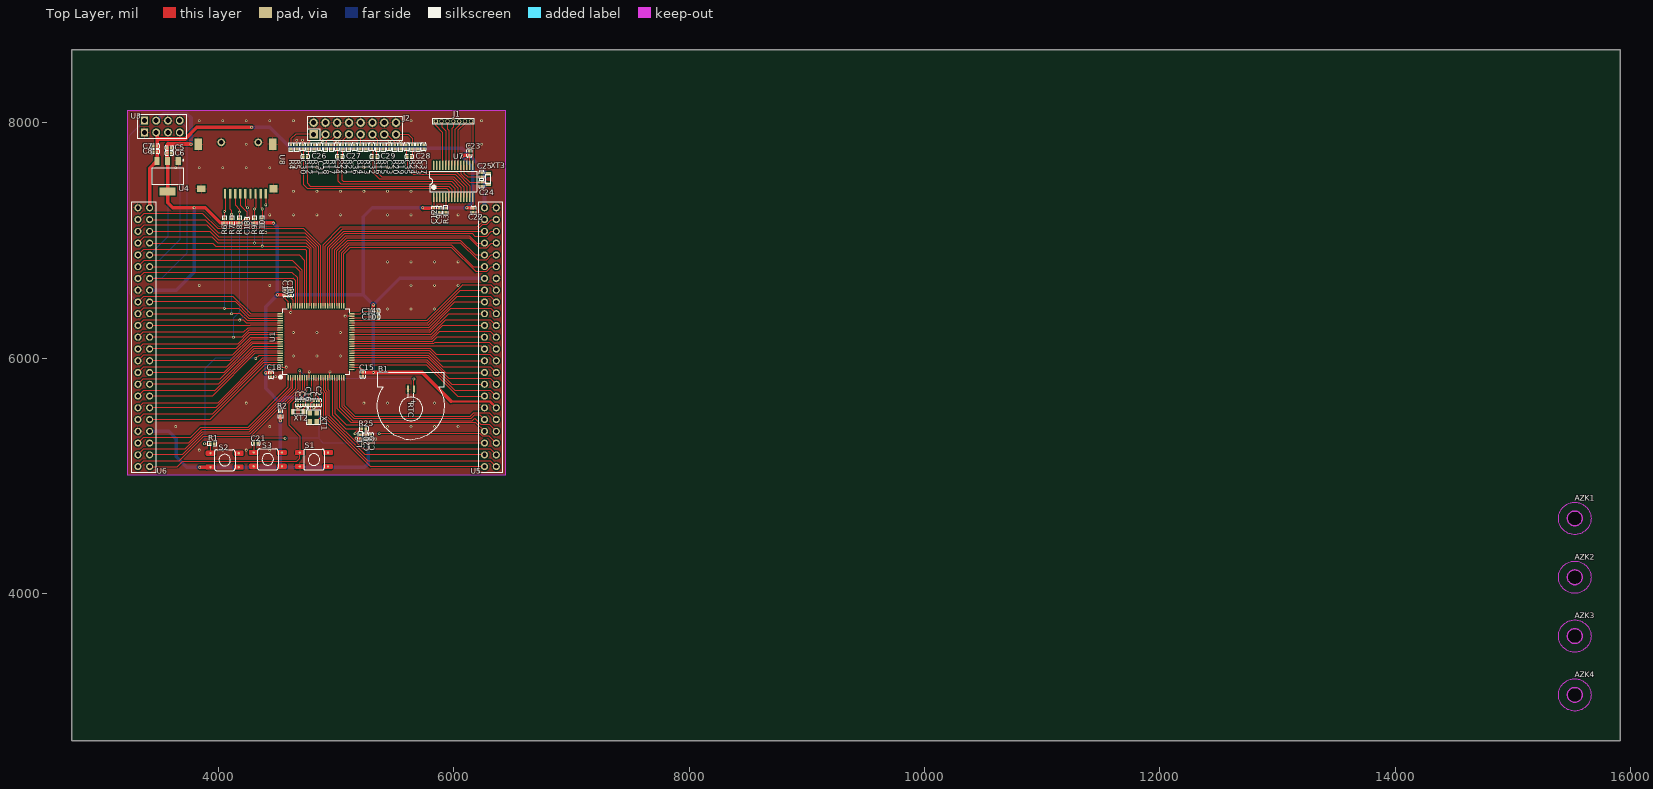
[diagram p0: Top Layer view]
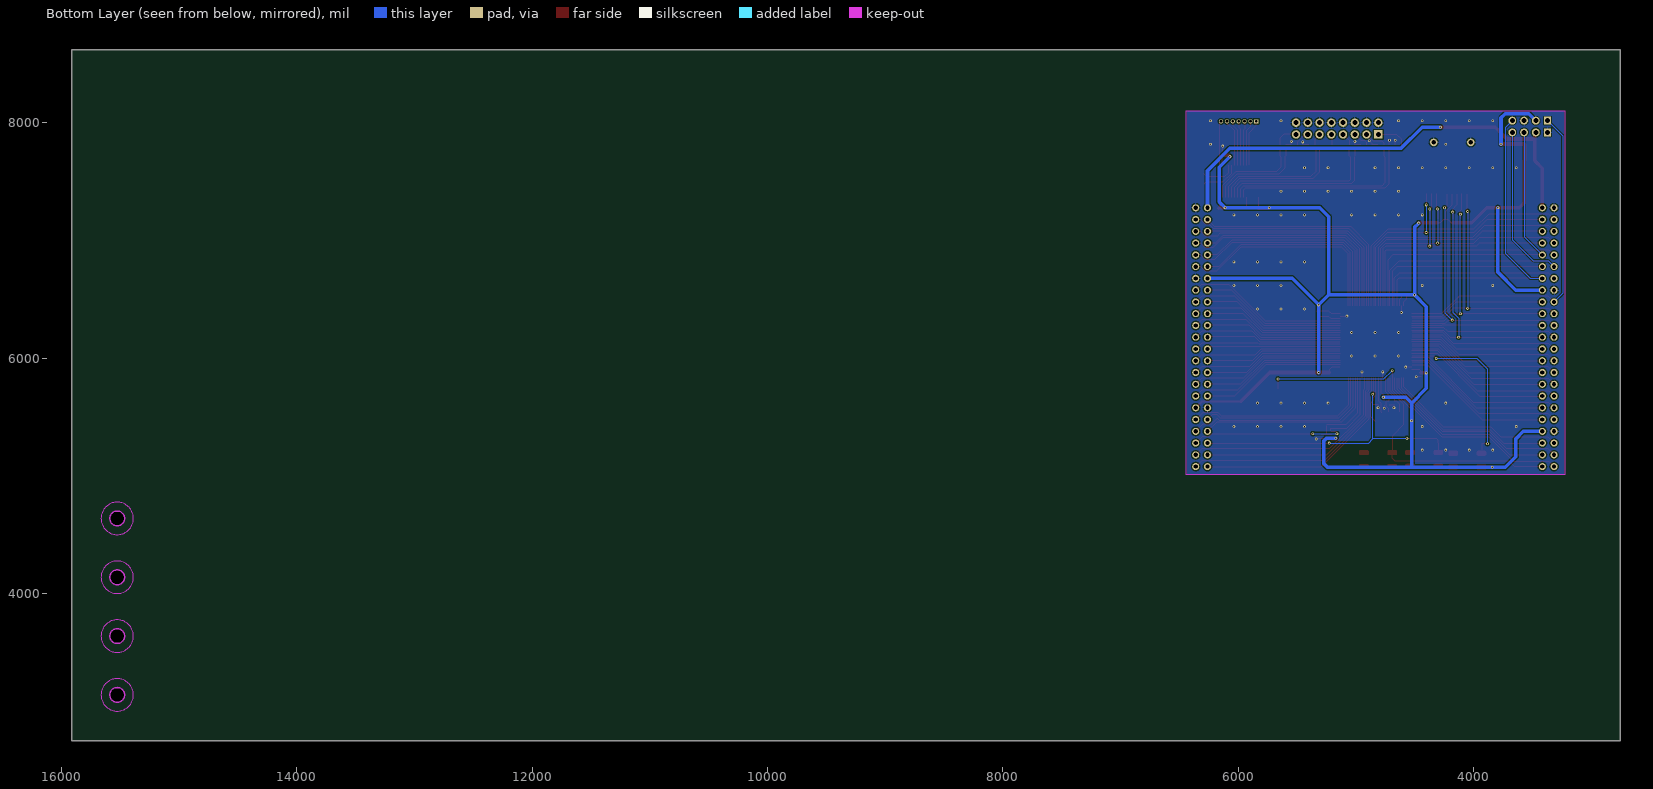
[diagram p1: Bottom Layer view, seen from below]
# Altium PCB MISC51975.pcbdoc
Units mil, origin at the board's own origin, x right, y up, seen from the top; angles counter-clockwise.
Board outline 13165.59 x 5873.19 mil, 2 copper layers (Top Layer, Bottom Layer), stack 2.757 mil thick; 83 components, 118 nets, 418 pads, 120 vias.

## Layer stack, top to bottom
Top Solder Mask Layer: solder mask 0.394, Dk 3.3
Top Layer: signal copper 1.379
Bottom Layer: signal copper 1.378
Bottom Solder Mask Layer: solder mask 0.394, Dk 3.3

## Board outline
15915.59,2750 2750,2750 2750,8623.19 15915.59,8623.19

## Design rules (kind name [scope] priority, off if disabled: settings)
BoardOutlineClearance Default_1 [All] p2: genericclearance=4 ignorepadtopadclearanceinfootprint=FALSE except(0: Arc-SplitContinuation Track-SplitContinuation SMDPad-SplitContinuation THPad-SplitContinuation Via-SplitContinuation Fill-SplitContinuation Region-SplitContinuation Poly-SplitContinuation Text-SplitContinuation Hole-SplitContinuation; 6: Arc-OutlineEdge Track-OutlineEdge SMDPad-OutlineEdge THPad-OutlineEdge Via-OutlineEdge Fill-OutlineEdge Region-OutlineEdge Poly-OutlineEdge Text-OutlineEdge Hole-OutlineEdge SMDPad-CutoutEdge THPad-CutoutEdge Via-CutoutEdge Fill-CutoutEdge Region-CutoutEdge Text-CutoutEdge; 6.9: Hole-CutoutEdge; 10: Poly-CutoutEdge; 11.8: Arc-CutoutEdge Track-CutoutEdge)
Clearance Default [All] p1: gap=4 ignorepadtopadclearanceinfootprint=FALSE except(6: SMDPad-Track SMDPad-SMDPad THPad-Track SMDPad-THPad THPad-THPad Track-Via SMDPad-Via THPad-Via Via-Via Fill-Track Region-Track Fill-SMDPad Region-SMDPad Fill-THPad Region-THPad Fill-Via Region-Via Fill-Fill Fill-Region Region-Region Arc-Track Arc-SMDPad Arc-THPad Arc-Via Fill-Arc Region-Arc Arc-Arc Text-Track SMDPad-Text Text-THPad Text-Via Fill-Text Region-Text Arc-Text Text-Text; 6.9: Hole-Track Hole-SMDPad Hole-THPad Hole-Via Fill-Hole Region-Hole Hole-Arc Hole-Text; 10: Poly-Track Poly-SMDPad Poly-THPad Poly-Via Poly-Fill Poly-Region Poly-Poly Poly-Arc Poly-Text Poly-Hole)
DiffPairsRouting differentialPair [All] p1: maxlimit=6 minlimit=5 mostfreqgap=6 toplayer_minwidth=5 toplayer_prefwidth=100 toplayer_maxwidth=100 toplayer_mingap=5 toplayer_prefgap=6 toplayer_maxgap=6 bottomlayer_minwidth=5 bottomlayer_prefwidth=100 bottomlayer_maxwidth=100 bottomlayer_mingap=5 bottomlayer_prefgap=6 bottomlayer_maxgap=6 maxuncoupledlength=10
HoleToHoleClearance otherClearance [All] p1: gap=11.8 allowstackedmicrovias=TRUE
Length netLength [All] p1: minlimit=0 maxlimit=0
MatchedLengths netLengthTolerance [All] p1: tolerance=1000
PasteMaskExpansion pasteMaskExpansion [All] p1: expansion=0
PlaneConnect innerPlane [All] p1: planeconnectstyle=Relief reliefexpansion=20 reliefentries=4 reliefconductorwidth=10 reliefairgap=10
PolygonConnect copperRegion [(InNet('GND'))] p1: connectstyle=Relief reliefconductorwidth=10 reliefentries=4 polygonreliefangle="90 Angle" airgapwidth=10 via.connectstyle=Relief via.reliefconductorwidth=10 via.reliefentries=4 via.polygonreliefangle="90 Angle" via.airgapwidth=10
RoutingVias Default_3 [All] p1: holewidth=12 width=24 viastyle="Through Hole" minholewidth=12 minwidth=24 maxholewidth=1181 maxwidth=1969
SolderMaskExpansion Common [IsVia] p1: expansion=-1000 istentingtop=TRUE
SolderMaskExpansion Common [All] p2: expansion=2 istentingtop=FALSE
Width Default_2 [All] p1: maxlimit=1000 minlimit=10 preferedwidth=10

## Components (designator, comment, footprint, x,y, rotation, side; value= is the part's Value field where it differs from the comment)
AZK1 "M3 mounting hole" M3安装孔(非金属化) 15527.8,4637.79 r0 top
AZK2 "M3 mounting hole" M3安装孔(非金属化) 15527.8,4137.79 r0 top
AZK3 "M3 mounting hole" M3安装孔(非金属化) 15527.8,3637.79 r0 top
AZK4 "M3 mounting hole" M3安装孔(非金属化) 15527.8,3137.79 r0 top
B1 "RTC" 焊盘引出RTC 5635.16,5567.96 r270 top
C1 "22pF" C0402 4808.14,5620.58 r90 top
C2 "22pF" C0402 4851.59,5621.23 r270 top
C3 "3pF" C0402 4673.14,5620.58 r270 top
C4 "3pF" C0402 4718.14,5620.58 r270 top
C5 "10uF" C0402 3580,7788.19 r180 top
C6 "10uF" C0402 3579.74,7741.59 r180 top
C7 "10uF" C0402 3459.74,7801.59 r180 top
C8 "100nF" C0402 3459.74,7756.59 r180 top
C9 "47uF" C0402 5875,7258.19 r90 top
C10 "100pF" C0402 5333.68,6351.39 r180 top
C11 "100pF" C0402 4613.68,6556.39 r270 top
C12 "100nF" C0402 5830,7258.19 r90 top
C13 "100pF" C0402 4240.52,7165.22 r90 top
C14 "100pF" C0402 5333.14,6400.58 r180 top
C15 "100pF" C0402 5225,5863.19 r90 top
C16 "100pF" C0402 4763.14,5620.58 r90 top
C17 "100pF" C0402 4568.14,6555.58 r270 top
C18 "100pF" C0402 4445,5858.19 r90 top
C19 "100pF" C0402 5293.66,5331.39 r90 top
C20 "10uF" C0402 5248.66,5330.88 r90 top
C21 "100nF" C0402 4316.73,5277.55 r180 top
C22 "47uF" C0402 6165,7258.19 r90 top
C23 "100nF" C0402 6130,7743.19 r270 top
C24 "47uF" C0402 6235,7478.19 r270 top
C25 "47uF" C0402 6235,7558.19 r90 top
C26 "10nF" C0402 4735,7713.19 r0 top
C27 "10nF" C0402 5030,7713.19 r0 top
C28 "10nF" C0402 5620,7713.19 r0 top
C29 "10nF" C0402 5325,7713.19 r0 top
C30 "1nF" C0402 4713.03,7795.67 r90 top
C31 "1nF" C0402 4860.1,7795.67 r90 top
C32 "1nF" C0402 5301.31,7795.67 r90 top
C33 "1nF" C0402 5448.38,7795.67 r90 top
C34 "1nF" C0402 5007.17,7795.67 r90 top
C35 "1nF" C0402 5595.45,7795.67 r90 top
C36 "1nF" C0402 5154.24,7795.67 r90 top
C37 "1nF" C0402 5742.52,7795.67 r90 top
J1 "1.27 pin header 7p" 1.27排针7P 6045,8013.19 r0 top
J2 "2.54 2*8P" HDR-TH_16P-P2.54-V-R2-C8-S2.54 5157.59,7952.11 r0 top
L1 "ferrite bead 600R" L0402 5203.14,5330.58 r90 top
R1 "10K" 贴片电阻0402封装 3945.92,5273.19 r0 top
R2 "200R" 贴片电阻0402封装 4525,5528.19 r90 top
R3 "0Ω" 贴片电阻0402封装 5930,7258.19 r90 top
R4 "100Ω" 贴片电阻0402封装 4615,7795.67 r270 top
R5 "10kΩ" 贴片电阻0402封装 4664,7795.67 r270 top
R6 "10K" 贴片电阻0402封装 4048.53,7167.99 r90 top
R7 "10K" 贴片电阻0402封装 4112.51,7167.99 r90 top
R8 "10K" 贴片电阻0402封装 4176.5,7167.99 r90 top
R9 "10K" 贴片电阻0402封装 4304.54,7167.99 r90 top
R10 "10K" 贴片电阻0402封装 4368.53,7167.99 r90 top
R11 "10kΩ" 贴片电阻0402封装 4811.07,7795.67 r270 top
R12 "100Ω" 贴片电阻0402封装 4762.07,7795.67 r270 top
R13 "10kΩ" 贴片电阻0402封装 5252.27,7795.67 r270 top
R14 "100Ω" 贴片电阻0402封装 5203.28,7795.67 r270 top
R15 "10kΩ" 贴片电阻0402封装 5399.34,7795.67 r270 top
R16 "100Ω" 贴片电阻0402封装 5350.35,7795.67 r270 top
R17 "10kΩ" 贴片电阻0402封装 4958.14,7795.67 r270 top
R18 "100Ω" 贴片电阻0402封装 4909.14,7795.67 r270 top
R19 "10kΩ" 贴片电阻0402封装 5546.41,7795.67 r270 top
R20 "100Ω" 贴片电阻0402封装 5497.42,7795.67 r270 top
R21 "10kΩ" 贴片电阻0402封装 5105.2,7795.67 r270 top
R22 "100Ω" 贴片电阻0402封装 5056.21,7795.67 r270 top
R23 "10kΩ" 贴片电阻0402封装 5693.48,7795.67 r270 top
R24 "100Ω" 贴片电阻0402封装 5644.49,7795.67 r270 top
R25 "0Ω" 贴片电阻0402封装 5233.14,5400.58 r180 top
S1 "K_USER" 按键开关4.5 4810,5138.19 r270 top
S2 "K_USER" 按键开关4.5 4051.41,5133.19 r270 top
S3 "K_USER" 按键开关4.5 4417.68,5139.98 r270 top
U1 "STM32H743VIT6" STM32H743VIT6 4828.14,6140.58 r90 top
U3 "HDR_2*4P" HDR_2*4P 3369.02,7919.17 r90 top
U4 "ASM1117" AMS1117-SOT-223 3566.29,7546.59 r180 top
U5 "STM32H7" 2*23 6310,6178.19 r180 top
U6 "STM32H7" 2*23 3363.54,6178.19 r180 top
U7 "ADS1256" SSOP-28_L10.2-W5.3-P0.65-LS7.8-BL 5994.95,7503.08 r0 top
U8 "MICRO SD TF card socket" "MICRO SD TF卡座" 4360.68,7507.71 r270 top
XT1 "XTAL3225" XTAL3225 4805,5498.19 r270 top
XT2 "32.768k" SMD-2012_2P 4675,5543.19 r0 top
XT3 "7.68MHz" SMD-2012_2P 6290,7523.19 r90 top

## Footprints (in the part's own frame and the unit in brackets; to place one, negate y for a bottom-side part, rotate by r counter-clockwise, add the part's x,y. Pads: shape width x height; smd on the part's side, far side on the other; paste and mask are expansions set on the pad)
1.27排针7P [mm]
  rect 0.9x0.9 hole 0.6 paste+0 mask+0.051: 1(-5.08,0)
  round 0.9 hole 0.6 paste+0 mask+0.051: 2(-3.81,0) 3(-2.54,0) 4(-1.27,0) 5(0,0) 6(1.27,0) 7(2.54,0)
  silkscreen extent -5.71,-0.64 3.17,0.64
2*23 [mil]
  round 60 hole 36 paste+0 mask+2: 1(-50,1100) 2(-50,1000) 3(-50,900) 4(-50,800) 5(-50,700) 6(-50,600) 7(-50,500) 8(-50,400) 9(-50,300) 10(-50,200) 11(-50,100) 12(-50,0) 13(-50,-100) 14(-50,-200) 15(-50,-300) 16(-50,-400) 17(-50,-500) 18(-50,-600) 19(-50,-700) 20(-50,-800) 21(-50,-900) 22(-50,-1000) 23(-50,-1100) 24(50,1100) 25(50,1000) 26(50,900) 27(50,800) 28(50,700) 29(50,600) 30(50,500) 31(50,400) 32(50,300) 33(50,200) 34(50,100) 35(50,0) 36(50,-100) 37(50,-200) 38(50,-300) 39(50,-400) 40(50,-500) 41(50,-600) 42(50,-700) 43(50,-800) 44(50,-900) 45(50,-1000) 46(50,-1100)
  silkscreen extent -100,-1150 100,1150
AMS1117-SOT-223 [mil]
  rect 43.3x68.9 smd paste+0 mask+2: 1(-90.55,-129.92) 2(0,-129.92) 3(90.55,-129.92)
  rect 137.79x68.9 smd paste+0 mask+2: 4(0,129.92)
  silkscreen extent -138,-143 132,73
C0402 [mm]
  rect 0.5x0.54 smd paste+0 mask+0.051: 1(-0.42,0) 2(0.42,0)
  silkscreen extent -0.87,-0.5 0.87,0.5
HDR-TH_16P-P2.54-V-R2-C8-S2.54 [mm]
  rect 1.8x1.8 hole 1.1 paste+0 mask+0.051: 1(-8.89,-1.27)
  round 1.8 hole 1.1 paste+0 mask+0.051: 2(-8.89,1.27) 3(-6.35,-1.27) 4(-6.35,1.27) 5(-3.81,-1.27) 6(-3.81,1.27) 7(-1.27,-1.27) 8(-1.27,1.27) 9(1.27,-1.27) 10(1.27,1.27) 11(3.81,-1.27) 12(3.81,1.27) 13(6.35,-1.27) 14(6.35,1.27) 15(8.89,-1.27) 16(8.89,1.27)
  silkscreen extent -10.3,-2.54 10.3,2.54
HDR_2*4P [mm]
  rect 1.7x1.524 hole 1.1 paste+0 mask+0.051: 1(0,0) 2(2.54,0)
  round 1.7 hole 1.1 paste+0 mask+0.051: 3(0,-2.54) 4(2.54,-2.54) 5(0,-5.08) 6(2.54,-5.08) 7(0,-7.62) 8(2.54,-7.62)
  silkscreen extent -1.4,-9.02 3.94,1.4
L0402 [mm]
  rect 0.54x0.54 smd paste+0 mask+0.051: 1(-0.42,0) 2(0.42,0)
  silkscreen extent -1.07,-0.51 1.07,0.49
M3安装孔(非金属化) [mil]
  Top Layer keep-out region: -137.8,0 -137.41,10.3 -136.26,20.54 -134.34,30.66 -131.67,40.62 -128.27,50.34 -124.15,59.79 -119.33,68.9 -113.85,77.62 -107.73,85.92 -101.01,93.73 -93.72,101.01 -85.91,107.73 -77.62,113.85 -68.9,119.34 -59.79,124.15 -50.34,128.27 -40.62,131.68 -30.66,134.34 -20.54,136.26 -10.3,137.41 0,137.8 10.3,137.41 20.54,136.26 30.66,134.34 40.62,131.68 50.34,128.27 59.79,124.15 68.9,119.34 77.62,113.85 85.91,107.73 93.72,101.01 101.01,93.73 107.73,85.92 113.85,77.62 119.33,68.9 124.15,59.79 128.27,50.34 131.67,40.62 134.34,30.66 136.26,20.54 137.41,10.3 137.8,0 137.41,-10.3 136.26,-20.54 134.34,-30.66 131.67,-40.61 128.27,-50.34 124.15,-59.78 119.33,-68.9 113.85,-77.62 107.73,-85.91 101.01,-93.72 93.72,-101.01 85.91,-107.73 77.62,-113.85 68.9,-119.33 59.79,-124.15 50.34,-128.27 40.62,-131.67 30.66,-134.34 20.54,-136.25 10.3,-137.41 0,-137.79 -10.3,-137.41 -20.54,-136.25 -30.66,-134.34 -40.62,-131.67 -50.34,-128.27 -59.79,-124.15 -68.9,-119.33 -77.62,-113.85 -85.91,-107.73 -93.72,-101.01 -101.01,-93.72 -107.73,-85.91 -113.85,-77.62 -119.33,-68.9 -124.15,-59.78 -128.27,-50.34 -131.67,-40.61 -134.34,-30.66 -136.26,-20.54 -137.41,-10.3
  Bottom Layer keep-out region: -137.8,0 -137.41,10.3 -136.26,20.54 -134.34,30.66 -131.67,40.62 -128.27,50.34 -124.15,59.79 -119.33,68.9 -113.85,77.62 -107.73,85.92 -101.01,93.73 -93.72,101.01 -85.91,107.73 -77.62,113.85 -68.9,119.34 -59.79,124.15 -50.34,128.27 -40.62,131.68 -30.66,134.34 -20.54,136.26 -10.3,137.41 0,137.8 10.3,137.41 20.54,136.26 30.66,134.34 40.62,131.68 50.34,128.27 59.79,124.15 68.9,119.34 77.62,113.85 85.91,107.73 93.72,101.01 101.01,93.73 107.73,85.92 113.85,77.62 119.33,68.9 124.15,59.79 128.27,50.34 131.67,40.62 134.34,30.66 136.26,20.54 137.41,10.3 137.8,0 137.41,-10.3 136.26,-20.54 134.34,-30.66 131.67,-40.61 128.27,-50.34 124.15,-59.78 119.33,-68.9 113.85,-77.62 107.73,-85.91 101.01,-93.72 93.72,-101.01 85.91,-107.73 77.62,-113.85 68.9,-119.33 59.79,-124.15 50.34,-128.27 40.62,-131.67 30.66,-134.34 20.54,-136.25 10.3,-137.41 0,-137.79 -10.3,-137.41 -20.54,-136.25 -30.66,-134.34 -40.62,-131.67 -50.34,-128.27 -59.79,-124.15 -68.9,-119.33 -77.62,-113.85 -85.91,-107.73 -93.72,-101.01 -101.01,-93.72 -107.73,-85.91 -113.85,-77.62 -119.33,-68.9 -124.15,-59.78 -128.27,-50.34 -131.67,-40.61 -134.34,-30.66 -136.26,-20.54 -137.41,-10.3
  Board Outline Layer circle w0.1: c0,0 r62.99
  Board Outline Layer region: 62.99,0 56.75,-27.33 39.27,-49.25 14.02,-61.41 -14.02,-61.41 -39.27,-49.25 -56.75,-27.33 -62.99,0 -62.99,0 -56.75,27.33 -39.27,49.25 -14.02,61.41 14.02,61.41 39.27,49.25 56.75,27.33 62.99,0
  Board Outline Layer region: 62.99,0 62.6,-7.05 61.41,-14.02 59.46,-20.8 56.75,-27.33 53.34,-33.51 49.25,-39.27 44.54,-44.54 39.27,-49.25 33.51,-53.34 27.33,-56.75 20.8,-59.46 14.02,-61.41 7.05,-62.6 0,-62.99 -7.05,-62.6 -14.02,-61.41 -20.8,-59.46 -27.33,-56.75 -33.51,-53.34 -39.27,-49.25 -44.54,-44.54 -49.25,-39.27 -53.34,-33.51 -56.75,-27.33 -59.46,-20.8 -61.41,-14.02 -62.6,-7.05 -62.99,0 -62.6,7.05 -61.41,14.02 -59.46,20.8 -56.75,27.33 -53.34,33.51 -49.25,39.27 -44.54,44.54 -39.27,49.25 -33.51,53.34 -27.33,56.75 -20.8,59.46 -14.02,61.41 -7.05,62.6 0,62.99 7.05,62.6 14.02,61.41 20.8,59.46 27.33,56.75 33.51,53.34 39.27,49.25 44.54,44.54 49.25,39.27 53.34,33.51 56.75,27.33 59.46,20.8 61.41,14.02 62.6,7.05
  Multi-Layer board cut-out: 62.99,0 56.75,-27.33 39.27,-49.25 14.02,-61.41 -14.02,-61.41 -39.27,-49.25 -56.75,-27.33 -62.99,0 -62.99,0 -56.75,27.33 -39.27,49.25 -14.02,61.41 14.02,61.41 39.27,49.25 56.75,27.33 62.99,0
"MICRO SD TF卡座" [mm]
  rect 2x0.5 smd paste+0 mask+0.051: 1(2.8,-7.784) 2(2.8,-6.684) 3(2.8,-5.584) 4(2.8,-4.484) 5(2.8,-3.384) 6(2.8,-2.284) 7(2.8,-1.184) 8(2.8,-0.084) 9(2.8,1.016)
  round 1.6 hole 1 paste+0 mask+0.051: 6(-8.3,-0.6) 6(-8.3,-8.6)
  rect 2.4x1.6 smd paste+0 mask+0.051: 6(-7.9,2.5) 6(-7.9,-13.6)
  rect 1.6x1.8 smd paste+0 mask+0.051: 6(1.7,2.7)
  rect 1.4x1.801 smd paste+0 mask+0.051: 6(1.7,-12.9)
SMD-2012_2P [mm]
  rect 0.8x1.2 smd paste+0 mask+0.051: 1(-1.157,0) 2(1.157,0)
  silkscreen extent -1.01,-0.51 0.99,0.5
SSOP-28_L10.2-W5.3-P0.65-LS7.8-BL [mm]
  oval 0.364x2.015 smd paste+0 mask+0.051: 1(-4.225,-3.455) 2(-3.575,-3.455) 3(-2.925,-3.455) 4(-2.275,-3.455) 5(-1.625,-3.455) 6(-0.975,-3.455) 7(-0.325,-3.455) 8(0.325,-3.455) 9(0.975,-3.455) 10(1.625,-3.455) 11(2.275,-3.455) 12(2.925,-3.455) 13(3.575,-3.455) 14(4.225,-3.455) 15(4.225,3.455) 16(3.575,3.455) 17(2.925,3.455) 18(2.275,3.455) 19(1.625,3.455) 20(0.975,3.455) 21(0.325,3.455) 22(-0.325,3.455) 23(-0.975,3.455) 24(-1.625,3.455) 25(-2.275,3.455) 26(-2.925,3.455) 27(-3.575,3.455) 28(-4.225,3.455)
  silkscreen extent -5.08,-2.2 5.08,2.2
STM32H743VIT6 [mm]
  oval 1.2x0.27 smd paste+0 mask+0.051: 1(-7.75,6) 2(-7.75,5.5) 3(-7.75,5) 4(-7.75,4.5) 5(-7.75,4) 6(-7.75,3.5) 7(-7.75,3) 8(-7.75,2.5) 9(-7.75,2) 10(-7.75,1.5) 11(-7.75,1) 12(-7.75,0.5) 13(-7.75,0) 14(-7.75,-0.5) 15(-7.75,-1) 16(-7.75,-1.5) 17(-7.75,-2) 18(-7.75,-2.5) 19(-7.75,-3) 20(-7.75,-3.5) 21(-7.75,-4) 22(-7.75,-4.5) 23(-7.75,-5) 24(-7.75,-5.5) 25(-7.75,-6) 51(7.75,-6) 52(7.75,-5.5) 53(7.75,-5) 54(7.75,-4.5) 55(7.75,-4) 56(7.75,-3.5) 57(7.75,-3) 58(7.75,-2.5) 59(7.75,-2) 60(7.75,-1.5) 61(7.75,-1) 62(7.75,-0.5) 63(7.75,0) 64(7.75,0.5) 65(7.75,1) 66(7.75,1.5) 67(7.75,2) 68(7.75,2.5) 69(7.75,3) 70(7.75,3.5) 71(7.75,4) 72(7.75,4.5) 73(7.75,5) 74(7.75,5.5) 75(7.75,6)
  oval 0.27x1.2 smd paste+0 mask+0.051: 26(-6,-7.75) 27(-5.5,-7.75) 28(-5,-7.75) 29(-4.5,-7.75) 30(-4,-7.75) 31(-3.5,-7.75) 32(-3,-7.75) 33(-2.5,-7.75) 34(-2,-7.75) 35(-1.5,-7.75) 36(-1,-7.75) 37(-0.5,-7.75) 38(0,-7.75) 39(0.5,-7.75) 40(1,-7.75) 41(1.5,-7.75) 42(2,-7.75) 43(2.5,-7.75) 44(3,-7.75) 45(3.5,-7.75) 46(4,-7.75) 47(4.5,-7.75) 48(5,-7.75) 49(5.5,-7.75) 50(6,-7.75) 76(6,7.75) 77(5.5,7.75) 78(5,7.75) 79(4.5,7.75) 80(4,7.75) 81(3.5,7.75) 82(3,7.75) 83(2.5,7.75) 84(2,7.75) 85(1.5,7.75) 86(1,7.75) 87(0.5,7.75) 88(0,7.75) 89(-0.5,7.75) 90(-1,7.75) 91(-1.5,7.75) 92(-2,7.75) 93(-2.5,7.75) 94(-3,7.75) 95(-3.5,7.75) 96(-4,7.75) 97(-4.5,7.75) 98(-5,7.75) 99(-5.5,7.75) 100(-6,7.75)
  silkscreen extent -7.7,-7.15 7.15,7.7
XTAL3225 [mm]
  rect 1.1x1 smd paste+0 mask+0.051: 1(-0.9,-0.75) 2(0.9,-0.75) 3(0.9,0.75) 4(-0.9,0.75)
  silkscreen extent -2.05,-1.43 1.67,1.48
按键开关4.5 [mm]
  round 0.5 smd: 1(-1.5,-3.05) 2(1.5,-3.05) 3(1.5,3.05) 4(-1.5,3.05)
  Top Layer region: -1.75,2.05 -1.774,2.051 -1.799,2.055 -1.823,2.061 -1.846,2.069 -1.868,2.08 -1.889,2.092 -1.909,2.107 -1.927,2.123 -1.943,2.141 -1.958,2.161 -1.97,2.182 -1.981,2.204 -1.989,2.227 -1.995,2.251 -1.999,2.275 -2,2.3 -2,3.8 -1.999,3.825 -1.995,3.849 -1.989,3.873 -1.981,3.896 -1.97,3.918 -1.958,3.939 -1.943,3.959 -1.927,3.977 -1.909,3.993 -1.889,4.008 -1.868,4.02 -1.846,4.031 -1.823,4.039 -1.799,4.045 -1.774,4.049 -1.75,4.05 -1.25,4.05 -1.225,4.049 -1.201,4.045 -1.177,4.039 -1.154,4.031 -1.132,4.02 -1.111,4.008 -1.091,3.993 -1.073,3.977 -1.057,3.959 -1.042,3.939 -1.03,3.918 -1.019,3.896 -1.011,3.873 -1.005,3.849 -1.001,3.825 -1,3.8 -1,2.3 -1.001,2.275 -1.005,2.251 -1.011,2.227 -1.019,2.204 -1.03,2.182 -1.042,2.161 -1.057,2.141 -1.073,2.123 -1.091,2.107 -1.111,2.092 -1.132,2.08 -1.154,2.069 -1.177,2.061 -1.201,2.055 -1.225,2.051 -1.25,2.05
  Top Layer region: 1.25,2.05 1.225,2.051 1.201,2.055 1.177,2.061 1.154,2.069 1.132,2.08 1.111,2.092 1.091,2.107 1.073,2.123 1.057,2.141 1.042,2.161 1.03,2.182 1.019,2.204 1.011,2.227 1.005,2.251 1.001,2.275 1,2.3 1,3.8 1.001,3.825 1.005,3.849 1.011,3.873 1.019,3.896 1.03,3.918 1.042,3.939 1.057,3.959 1.073,3.977 1.091,3.993 1.111,4.008 1.132,4.02 1.154,4.031 1.177,4.039 1.201,4.045 1.225,4.049 1.25,4.05 1.75,4.05 1.774,4.049 1.799,4.045 1.823,4.039 1.846,4.031 1.868,4.02 1.889,4.008 1.909,3.993 1.927,3.977 1.943,3.959 1.958,3.939 1.97,3.918 1.981,3.896 1.989,3.873 1.995,3.849 1.999,3.825 2,3.8 2,2.3 1.999,2.275 1.995,2.251 1.989,2.227 1.981,2.204 1.97,2.182 1.958,2.161 1.943,2.141 1.927,2.123 1.909,2.107 1.889,2.092 1.868,2.08 1.846,2.069 1.823,2.061 1.799,2.055 1.774,2.051 1.75,2.05
  Top Layer region: -1.75,-4.05 -1.774,-4.049 -1.799,-4.045 -1.823,-4.039 -1.846,-4.031 -1.868,-4.02 -1.889,-4.008 -1.909,-3.993 -1.927,-3.977 -1.943,-3.959 -1.958,-3.939 -1.97,-3.918 -1.981,-3.896 -1.989,-3.873 -1.995,-3.849 -1.999,-3.825 -2,-3.8 -2,-2.3 -1.999,-2.276 -1.995,-2.251 -1.989,-2.227 -1.981,-2.204 -1.97,-2.182 -1.958,-2.161 -1.943,-2.141 -1.927,-2.123 -1.909,-2.107 -1.889,-2.092 -1.868,-2.08 -1.846,-2.069 -1.823,-2.061 -1.799,-2.055 -1.774,-2.051 -1.75,-2.05 -1.25,-2.05 -1.225,-2.051 -1.201,-2.055 -1.177,-2.061 -1.154,-2.069 -1.132,-2.08 -1.111,-2.092 -1.091,-2.107 -1.073,-2.123 -1.057,-2.141 -1.042,-2.161 -1.03,-2.182 -1.019,-2.204 -1.011,-2.227 -1.005,-2.251 -1.001,-2.276 -1,-2.3 -1,-3.8 -1.001,-3.825 -1.005,-3.849 -1.011,-3.873 -1.019,-3.896 -1.03,-3.918 -1.042,-3.939 -1.057,-3.959 -1.073,-3.977 -1.091,-3.993 -1.111,-4.008 -1.132,-4.02 -1.154,-4.031 -1.177,-4.039 -1.201,-4.045 -1.225,-4.049 -1.25,-4.05
  Top Layer region: 1.25,-4.05 1.225,-4.049 1.201,-4.045 1.177,-4.039 1.154,-4.031 1.132,-4.02 1.111,-4.008 1.091,-3.993 1.073,-3.977 1.057,-3.959 1.042,-3.939 1.03,-3.918 1.019,-3.896 1.011,-3.873 1.005,-3.849 1.001,-3.825 1,-3.8 1,-2.3 1.001,-2.276 1.005,-2.251 1.011,-2.227 1.019,-2.204 1.03,-2.182 1.042,-2.161 1.057,-2.141 1.073,-2.123 1.091,-2.107 1.111,-2.092 1.132,-2.08 1.154,-2.069 1.177,-2.061 1.201,-2.055 1.225,-2.051 1.25,-2.05 1.75,-2.05 1.774,-2.051 1.799,-2.055 1.823,-2.061 1.846,-2.069 1.868,-2.08 1.889,-2.092 1.909,-2.107 1.927,-2.123 1.943,-2.141 1.958,-2.161 1.97,-2.182 1.981,-2.204 1.989,-2.227 1.995,-2.251 1.999,-2.276 2,-2.3 2,-3.8 1.999,-3.825 1.995,-3.849 1.989,-3.873 1.981,-3.896 1.97,-3.918 1.958,-3.939 1.943,-3.959 1.927,-3.977 1.909,-3.993 1.889,-4.008 1.868,-4.02 1.846,-4.031 1.823,-4.039 1.799,-4.045 1.774,-4.049 1.75,-4.05
  silkscreen extent -2.25,-2.25 2.25,2.25
焊盘引出RTC [mil]
  rect 60x20 smd paste+0 mask+2: 1(-170,25) 2(-170,-25)
  silkscreen extent -311,-287 264,282
贴片电阻0402封装 [mm]
  rect 0.566x0.54 smd paste-100 mask+0.051: 1(-0.433,0) 2(0.433,0)
  silkscreen extent -0.94,-0.5 0.94,0.5

## Via types
v1: diameter 24, hole 12, Top Layer to Bottom Layer, 65 vias
v2: diameter 24.02, hole 12, Top Layer to Bottom Layer, 55 vias

## Nets (pads, with @x,y where several pads share a name; then routed paths per layer and width w, separated by ;. In a path a pad name is that pad's centre, name@x,y a point inside that pad or via, vN(x,y) a via of type N, cw(c..) or ccw(c..) an arc to the next point about the centre after c; other vN are vias at no path point)
3V3: C5.2 C6.2 C9.2 C12.2 C13.2 C14.2 C15.2 C16.2 C17.2 C18.2 C22.2 C23.2 L1.1 R2.1 R6.1 R7.1 R8.1 R9.1 R10.1 S2.2 U1.11 U1.27 U1.50 U1.75 U1.100 U3.4 U4.2 U4.4 U5.6 U5.40 U6.4 U6.16 U7.1 U7.14 U7.16 U8.4 | length 15705.7
  Top Layer w10: R8.1 4187.76,7150.95 4218.57,7181.76 C13.2 ; U8.4 4184.14,7299.06 4240.52,7242.67 C13.2 ; R9.1 4282.24,7150.95 4251.43,7181.76 C13.2 ; C18.2 4445,5889.36 4460,5904.36 U1.100 ; C17.2 4568.14,6505.06 4591.92,6481.27 U1.75 ; C16.2 4763.77,5637.75 4763.77,5686.96 4788.77,5711.96 U1.11 ; U1.27 5204.15,5924.04 5225,5903.19 C15.2 ; U1.50 5203.61,6376.8 5227.38,6400.58 C14.2 ; U7.1 5830,7365.67 C12.2 C9.2 ; C23.2 6135.7,7720.95 U7.16 ; C22.2@6161.29,7278.44 U7.14
  Top Layer w20: 5976,5632.19 6306,5632.19 U5.6
  Top Layer w30: v2(3765,7818.19) 3762.55,7820.64 3569.19,7820.64 3563.46,7814.91 C5.2 3563.46,7679.33 U4.2 U4.4 3566.29,7321.9 3610,7278.19 v2(3791.09,7278.19) 3885,7278.19 4012.24,7150.95 R6.1 R7.1 R8.1 ; v2(3840,5073.19) 3930.39,5073.19 S2.2 ; R9.1 R10.1 4462.24,7150.95 v2(4465,7148.19) ; v2(4400,5874.82) 4444.91,5874.82 C18.2 ; v2(4500,6538.19) 4567.29,6538.19 C17.2 ; v2(4525,5468.19) R2.1 ; v2(5170,5319.41) 5175.36,5314.05 L1.1 ; C15.2 5226.54,5878.19 v2(5315,5878.19) 5730,5878.19 5976,5632.19 ; v2(5315,6453.19) 5315,6402.17 C14.2 ; v2(5735,7278.19) 5738.46,7274.73 C12.2 ; v2(6070,7713.19) 6083.46,7726.65 C23.2 ; v2(6110,7278.19) 6161.54,7278.19 C22.2
  Bottom Layer w30: U6.4 3575,5378.19 3640,5313.19 3640,5163.19 3730,5073.19 v2(3840,5073.19) 4525.06,5073.19 5240,5073.19 5270,5103.19 5270,5298.19 5248.79,5319.41 v2(5170,5319.41) ; U6.16 3640,6578.19 3791.09,6729.28 v2(3791.09,7278.19) ; U3.4 3528.04,8078.19 3730,8078.19 3765,8043.19 v2(3765,7818.19) ; v2(4465,7148.19) 4500,7113.19 v2(4500,6538.19) ; 4525,5073.25 v2(4525,5468.19) 4525,5618.19 ; v2(4765,5668.19) 4575,5668.19 4525,5618.19 ; v2(5315,5878.19) v2(5315,6453.19) ; v2(6070,7713.19) 6160,7623.19 6160,7328.19 v2(6110,7278.19) v2(5735,7278.19) 5305,7278.19 5230,7203.19 5230,6538.19 ; U5.40 5540,6678.19 v2(5315,6453.19) ; v2(4500,6538.19) 4400,6438.19 v2(4400,5874.82) 4400,5743.19 4525,5618.19 ; v2(4500,6538.19) 5230,6538.19 ; 5230,6538.19 v2(5315,6453.19)
5V: C7.1 C8.1 U3.3 U4.3 U5.46 U6.23 | length 3963.4
  Top Layer w30: U6.23 3413.54,7614.31 U4.3 3476.28,7677.04 C8.1 C7.1 3476.28,7863.19 ; U3.3 3476.28,7911.92 3476.28,7863.19 ; v2(4280,7963.19) 3815,7963.19 3715,7863.19 3476.28,7863.19
  Bottom Layer w30: v2(4280,7963.19) 4435,7963.19 4615,7783.19 6070,7783.19 6260,7593.19 U5.46
$2N245: R3.2 U7.5 | length 92.2
  Top Layer w10: R3.2 5930.97,7276.2 U7.5
$2N255: J1.7 U7.15 | length 380.8
  Top Layer w10: J1.7 6161.29,7996.9 U7.15
$2N260: J1.6 U7.20 | length 399.6
  Top Layer w10: U7.20 6033.34,7936.53 6095,7998.19 J1.6
$2N261: J1.5 U7.21 | length 389.5
  Top Layer w10: U7.21@6007.75,7639.11 6007.75,7940.94 6045,7978.19 J1.5
$2N262: J1.4 U7.22 | length 379.4
  Top Layer w10: U7.22 5982.16,7950.35 5995,7963.19 J1.4
$2N263: J1.3 U7.23 | length 378.9
  Top Layer w10: J1.3 5945,7948.19 5956.56,7936.63 U7.23
$2N264: J1.2 U7.24 | length 389
  Top Layer w10: J1.2 5895,7968.19 5930.97,7932.22 U7.24
$2N265: J1.1 U7.25 | length 399.1
  Top Layer w10: J1.1 5845,7978.19 5905.38,7917.81 U7.25
BOOT0: R1.1 S2.1 U1.94 | length 1456.2
  Top Layer w10: v2(3880,5273.19) R1.1 3928.88,5194.7 S2.1@3931.33,5192.25 ; v2(4315,5998.19) 4339.28,6022.47 U1.94
  Bottom Layer w10: v2(3880,5273.19) 3880,5908.19 3970,5998.19 v2(4315,5998.19)
CH0: C26.1 C30.1 R4.2 R5.2 U7.6 | length 1719.6
  Top Layer w10: R4.2 R5.2 4712.53,7778.63 C30.1 4718.46,7773.7 C26.1 4718.46,7479.73 4755,7443.19 5940,7443.19 5956.56,7426.63 U7.6
CH1: C26.2 C31.1 R11.2 R12.2 U7.7 | length 1712.2
  Top Layer w10: C31.1 4859.6,7778.63 R11.2 R12.2 4762.07,7723.72 C26.2 4751.54,7491.65 4780,7463.19 5955,7463.19 5982.16,7436.03 U7.7
CH2: C27.1 C34.1 R17.2 R18.2 U7.8 | length 1469.5
  Top Layer w10: R18.2 R17.2 5006.67,7778.63 C34.1 5007.17,7719.48 C27.1 5013.46,7509.73 5040,7483.19 5970,7483.19 6007.75,7445.44 U7.8@6007.75,7367.05
CH3: C27.2 C36.1 R21.2 R22.2 U7.9 | length 1461.5
  Top Layer w10: C36.1 5153.74,7778.63 R21.2 R22.2 5056.21,7722.86 C27.2 5046.54,7516.65 5060,7503.19 5980,7503.19 6033.34,7449.85 U7.9
CH4: C29.1 C32.1 R13.2 R14.2 U7.10 | length 1190.2
  Top Layer w10: R14.2 R13.2 5300.81,7778.63 C32.1 5308.46,7771.98 C29.1 5308.46,7579.73 5365,7523.19 5990,7523.19 6058.93,7454.26 U7.10
CH5: C29.2 C33.1 R15.2 R16.2 U7.11 | length 1181.5
  Top Layer w10: C33.1 5447.88,7778.63 R15.2 R16.2 5341.54,7769.82 C29.2 5341.54,7586.65 5385,7543.19 6000,7543.19 6084.52,7458.67 U7.11
CH6: C28.1 C35.1 R19.2 R20.2 U7.12 | length 931.4
  Top Layer w10: R20.2 R19.2 5594.95,7778.63 C35.1 5595.45,7721.2 C28.1 5603.46,7614.73 5655,7563.19 6010,7563.19 6110.11,7463.08 U7.12
CH7: C28.2 C37.1 R23.2 R24.2 U7.13 | length 922
  Top Layer w10: C37.1 5742.02,7778.63 R23.2 R24.2 5644.49,7721.14 C28.2 5636.54,7621.65 5675,7583.19 6020,7583.19 6135.7,7467.49 U7.13
GND: B1.2 C1.1 C2.2 C3.2 C4.2 C5.1 C6.1 C7.2 C8.2 C9.1 C10.1 C11.1 C12.1 C13.1 C14.1 C15.1 C16.1 C17.1 C18.1 C19.1 C20.1 C21.1 C22.1 C23.1 C24.2 C25.2 C30.2 C31.2 C32.2 C33.2 C34.2 C35.2 C36.2 C37.2 J2.2 J2.4 J2.6 J2.8 J2.10 J2.12 J2.14 J2.16 R1.2 R3.1 R5.1 R11.1 R13.1 R15.1 R17.1 R19.1 R21.1 R23.1 S1.2 S3.2 U1.10 U1.19 U1.26 U1.49 U1.74 U1.99 U3.1 U3.6 U4.1 U5.17 U5.23 U5.29 U6.27 U6.39 U6.46 U7.2 U7.3 U7.17 U8.6 XT1.2 XT1.4 | length 1021.4
  Top Layer w10: C18.1 v2(4485,5841.65) ; U1.99 v2(4575,5924.04) ; v2(4611.6,6388.19) U1.74 ; R5.1 v2(4664,7853.19) ; v2(4675,5578.19) 4675,5602.17 C3.2 C4.2 ; C30.2 v2(4713.03,7853.19) ; v2(4757,5574.33) 4757,5597.9 C16.1 ; U1.10 4770,5836.38 v2(4770,5883.19) ; v2(4810,5578.19) 4810,5602.17 C1.1 4850.94,5604.04 C2.2 ; R11.1 4859.6,7812.71 C31.2 4860.1,7822.08 v2(4885.61,7847.59) ; U1.19@4946.25,5835.46 v2(4946.25,5883.19) ; R17.1 5006.67,7812.71 C34.2 v2(5007.17,7843.19) ; v2(5075,6358.19) 5132.17,6358.19 U1.49 ; C20.1 5293.15,5314.34 C19.1 5333.34,5314.85 v2(5335,5313.19) ; R15.1 5447.88,7812.71 C33.2 5450,7813.82 v2(5450,7838.19) ; v2(5546.41,7843.19) R19.1 5594.95,7812.71 C35.2 ; C23.1 v2(6130,7803.19)
  other v1: 3835.1,5218.29 4035.1,5218.29 4235.1,5218.29 4435.1,5218.29 3635.1,5418.29 4435.1,5418.29 5435.1,5418.29 5635.1,5418.29 5835.1,5418.29 6035.1,5418.29 4235.1,5618.29 5235.1,5618.29 5435.1,5618.29 5635.1,5618.29 5835.1,5618.29 4635.1,6018.29 4835.1,6018.29 5035.1,6018.29 4635.1,6218.29 4835.1,6218.29 5035.1,6218.29 5435.1,6418.29 5635.1,6418.29 5835.1,6418.29 3835.1,6618.29 4435.1,6618.29 5635.1,6618.29 5835.1,6618.29 6035.1,6618.29 5435.1,6818.29 5635.1,6818.29 5835.1,6818.29 6035.1,6818.29 4435.1,7218.29 4635.1,7218.29 4835.1,7218.29 5035.1,7218.29 5435.1,7218.29 5635.1,7218.29 5835.1,7218.29 6035.1,7218.29 4635.1,7418.29 4835.1,7418.29 5035.1,7418.29 5235.1,7418.29 5435.1,7418.29 5635.1,7418.29 3635.1,7618.29 3835.1,7618.29 4035.1,7618.29 4235.1,7618.29 4435.1,7618.29 4635.1,7618.29 4835.1,7618.29 5235.1,7618.29 5435.1,7618.29 4235.1,7818.29 6235.1,7818.29 3835.1,8018.29 4035.1,8018.29 4235.1,8018.29 4435.1,8018.29 4635.1,8018.29 5635.1,8018.29 6235.1,8018.29
IN0: J2.1 R4.1 | length 259.2
  Top Layer w10: R4.1 4615,7863.19 4653.92,7902.11 J2.1
IN1: J2.3 R12.1 | length 192.8
  Top Layer w10: R12.1 4762.07,7830.26 4780,7848.19 4853.68,7848.19 J2.3
IN2: J2.5 R18.1 | length 149.9
  Top Layer w10: R18.1 4909.14,7837.33 4925,7853.19 4958.68,7853.19 J2.5
IN3: J2.7 R22.1 | length 110.7
  Top Layer w10: R22.1 5056.21,7850.73 J2.7
IN4: J2.9 R14.1 | length 91.2
  Top Layer w10: R14.1 5203.28,7897.8 J2.9
IN5: J2.11 R16.1 | length 107.1
  Top Layer w10: J2.11 5350.35,7859.36 R16.1
IN6: J2.13 R20.1 | length 140.4
  Top Layer w10: J2.13 5431.08,7902.11 5497.42,7835.77 R20.1
IN7: J2.15 R24.1 | length 206.7
  Top Layer w10: J2.15 5611.08,7902.11 5644.49,7868.71 R24.1
NRST: C21.2 S3.1 U1.14 U5.26 | length 2611.8
  Top Layer w10: S3.1 4300.19,5201.63 C21.2 4300.19,5301 4317.38,5318.19 v2(4565,5318.19) ; U1.14 4847.82,5700.37 v2(4855,5693.19) ; v2(5225,5278.19) U5.26
  Bottom Layer w10: v2(4565,5318.19) 4850,5318.19 4855,5313.19 ; v2(4855,5693.19) 4855,5313.19 ; v2(5225,5278.19) 4890,5278.19 4855,5313.19
OSC_IN_H: C1.2 U1.12 XT1.1 | length 317.2
  Top Layer w10: XT1.1 4785,5543.15 4785,5616.93 4792.95,5624.88 4795.9,5624.88 C1.2 4808.14,5789.43 4808.45,5789.74 U1.12
OSC_IN_L: C3.1 U1.8 XT2.1 | length 345.1
  Top Layer w10: XT2.1 4629.45,5612.65 4653.92,5637.12 C3.1 4673.14,5666.33 4729.71,5722.9 U1.8
OSC_OUT_H: C2.1 U1.13 XT1.3 | length 410.1
  Top Layer w10: U1.13 4828.14,5685.05 4851.59,5661.6 C2.1 4854.54,5637.77 4874.35,5617.95 4874.35,5502.59 XT1.3
OSC_OUT_L: C4.1 U1.9 XT2.2 | length 333.7
  Top Layer w10: XT2.2 4720.55,5570.42 4740,5589.87 4740,5633.19 4735,5638.19 4719.21,5638.19 C4.1 4718.14,5686.33 4749.4,5717.59 U1.9
PA0: U1.22 U5.27 | length 1598.4
  Top Layer w10: U1.22 5005.3,5574.37 5124.85,5454.82 6162.01,5454.82 6163.67,5456.48 6181.72,5456.48 U5.27
PA1: U1.23 U5.4 | length 1689.1
  Top Layer w10: U1.23 5024.99,5582.52 5138.69,5468.82 6156.22,5468.82 6176.2,5488.81 6227.82,5437.19 6301,5437.19 U5.4
PA2: U1.24 U5.28 | length 1531.1
  Top Layer w10: U1.24 5044.67,5590.68 5146.84,5488.5 6148.06,5488.5 6177.57,5518.01 6220.18,5518.01 U5.28
PA3: U1.25 U5.5 | length 1606.3
  Top Layer w10: U1.25 5064.36,5598.83 5155,5508.19 6139.91,5508.19 6168.91,5537.19 6301,5537.19 U5.5
PA4: U1.28 U5.30 | length 1236.7
  Top Layer w10: U1.28 5765,5943.73 6030.54,5678.19 U5.30
PA5: U1.29 U5.7 | length 1344.9
  Top Layer w10: U1.29 5769.78,5963.41 6005,5728.19 6310,5728.19 U5.7
PA6: U1.30 U5.31 | length 1211.6
  Top Layer w10: U1.30 5775.09,5983.1 5980,5778.19 U5.31
PA7: U1.31 U5.8 | length 1319.8
  Top Layer w10: U1.31 5780.41,6002.78 5955,5828.19 6310,5828.19 U5.8
PA8: U1.67 U6.42 | length 1926.1
  Top Layer w10: U6.42 3358.54,6923.19 4739.4,6923.19 4749.4,6913.19 U1.67
PA9: U1.68 U3.5 U6.19 | length 2827.9
  Top Layer w10: U6.19 4685,6878.19 4729.71,6833.48 U1.68
  Bottom Layer w10: U6.19 3569.02,7033.67 U3.5
PA10: U1.69 U3.7 U6.41 | length 3115.1
  Top Layer w10: U6.41 3363.54,6828.19 4630,6828.19 4710.03,6748.16 U1.69
  Bottom Layer w10: U6.41 3363.54,6828.19 3490,6828.19 3669.02,7007.22 U3.7
PA11: U1.70 U6.18 | length 1585.7
  Top Layer w10: U6.18 4650,6778.19 4690.34,6737.85 U1.70
PA12: U1.71 U6.40 | length 1633.6
  Top Layer w10: U6.40 3363.54,6728.19 4625,6728.19 4670.66,6682.53 U1.71
PA15: U1.77 U6.15 | length 1159.6
  Top Layer w10: U6.15 4145,6478.19 4266.08,6357.11 U1.77
PB0: U1.34 U5.33 | length 1161.4
  Top Layer w10: U1.34 5796.35,6061.84 5880,5978.19 U5.33
PB1: U1.35 U5.10 | length 1269.5
  Top Layer w10: U1.35 5801.67,6081.52 5855,6028.19 6310,6028.19 U5.10
PB2: U1.36 U5.34 | length 1136.3
  Top Layer w10: U1.36 6236.98,6101.21 U5.34
PB3: U1.89 U6.9 | length 1210
  Top Layer w10: U6.9 4045,5878.19 4287.7,6120.89 U1.89
PB4: U1.90 U6.31 | length 1343.3
  Top Layer w10: U6.31 3358.54,5823.19 4015,5823.19 4293.02,6101.21 U1.90
PB5: U1.91 U6.8 | length 1235.1
  Top Layer w10: U6.8 3995,5778.19 4298.33,6081.52 U1.91
PB6: U1.92 U6.30 | length 1368.4
  Top Layer w10: U6.30 3358.54,5723.19 3965,5723.19 4303.65,6061.84 U1.92
PB7: U1.93 U6.7 | length 1260.2
  Top Layer w10: U6.7 3945,5678.19 4308.96,6042.15 U1.93
PB8: U1.95 U6.29 | length 1385.3
  Top Layer w10: U6.29 3358.54,5623.19 3995,5623.19 4374.59,6002.78 U1.95
PB9: U1.96 U6.6 | length 1277.2
  Top Layer w10: U6.6 3975,5578.19 4379.91,5983.1 U1.96
PB10: U1.46 U5.39 | length 1242.8
  Top Layer w10: U1.46 5774.87,6298.06 6055,6578.19 U5.39
PB11: U1.47 U5.16 | length 1371.9
  Top Layer w10: U1.47 5769.55,6317.74 6075,6623.19 6315,6623.19 U5.16
PB12: U1.51 U5.18 | length 1862.9
  Top Layer w10: U1.51 5064.36,6887.55 5120,6943.19 5978.13,6943.19 6184.13,6737.19 6276.98,6737.19 6317.98,6778.19 U5.18
PB13: U1.52 U5.41 | length 1769.7
  Top Layer w10: U1.52 5044.67,6895.71 5111.84,6962.88 5978.24,6962.88 6162.93,6778.19 U5.41
PB14: U1.53 U5.19 | length 1903
  Top Layer w10: U1.53 5024.99,6903.86 5103.69,6982.56 6055.06,6982.56 6200.43,6837.19 6276.98,6837.19 6317.98,6878.19 U5.19
PB15: U1.54 U5.42 | length 1809.8
  Top Layer w10: U1.54 5005.3,6912.02 5095.54,7002.25 6055.17,7002.25 6179.23,6878.19 U5.42
PC0: U1.15 U5.24 | length 1901.4
  Top Layer w10: U1.15 4867.51,5720.68 4888.35,5699.84 4888.35,5481.33 5291.49,5078.19 U5.24
PC1: U1.16 U5.1 | length 1976.9
  Top Layer w10: U1.16 4887.19,5726 4905,5708.19 4905,5492.52 5269.32,5128.19 6310,5128.19 U5.1
PC2: U1.17 U5.25 | length 1811.1
  Top Layer w10: U1.17 4906.88,5731.31 4920,5718.19 4920,5505.36 5247.17,5178.19 U5.25
PC3: U1.18 U5.2 | length 1886.6
  Top Layer w10: U1.18 4926.56,5736.63 4936.56,5726.63 4936.56,5516.63 5225,5228.19 6310,5228.19 U5.2
PC4: U1.32 U5.32 | length 1186.5
  Top Layer w10: U1.32 5785.72,6022.47 5930,5878.19 U5.32
PC5: U1.33 U5.9 | length 1294.7
  Top Layer w10: U1.33 5791.04,6042.15 5905,5928.19 6310,5928.19 U5.9
PC6: U1.63 U6.44 | length 2110.5
  Top Layer w10: U6.44 3363.54,7128.19 3905,7128.19 4005,7028.19 4745,7028.19 4828.14,6945.05 U1.63
PC7: U1.64 U6.21 | length 1946.3
  Top Layer w10: U6.21 3925,7078.19 3995,7008.19 4740,7008.19 4808.45,6939.74 U1.64
PC8: R9.2 U1.65 U6.43 U8.7 | length 2529.4
  Top Layer w10: U6.43 3363.54,7028.19 3945,7028.19 3995,6978.19 v2(4304.54,6978.19) 4745,6978.19 4788.77,6934.42 U1.65 ; R9.2 v2(4304.54,7267.74) 4314.07,7277.26 U8.7
  Bottom Layer w10: v2(4304.54,6978.19) v2(4304.54,7267.74)
PC9: R10.2 U1.66 U6.20 U8.8 | length 2392.6
  Top Layer w10: U6.20 3950,6978.19 3975,6953.19 v2(4370,6953.19) 4745,6953.19 4769.08,6929.11 U1.66 ; U8.8 4357.37,7280.83 v2(4370,7268.19) 4370,7186.5 R10.2
  Bottom Layer w10: v2(4370,6953.19) v2(4370,7268.19)
PC10: R6.2 U1.78 U6.37 U8.1 | length 2302
  Top Layer w10: U6.37 3358.54,6423.19 v2(4048.53,6423.19) 4170,6423.19 4255.76,6337.43 U1.78 ; R6.2 v2(4048.53,7246.72) 4054.22,7252.41 U8.1
  Bottom Layer w10: v2(4048.53,6423.19) v2(4048.53,7246.72)
PC11: R7.2 U1.79 U6.14 U8.2 | length 2198.2
  Top Layer w10: U6.14 v2(4110,6378.19) 4185,6378.19 4245.45,6317.74 U1.79 ; U8.2 4097.53,7265.67 4110,7253.19 v2(4110,7223.19) 4110,7187.54 R7.2
  Bottom Layer w10: v2(4110,6378.19) v2(4110,7223.19)
PC12: U1.80 U6.36 U8.5 | length 2347
  Top Layer w10: U6.36 3358.54,6323.19 v2(4180,6323.19) 4215,6323.19 4240.13,6298.06 U1.80 ; U8.5 4227.45,7295.75 v2(4245,7278.19)
  Bottom Layer w10: v2(4180,6323.19) 4245,6388.19 v2(4245,7278.19)
PC13: S1.1 U1.7 U6.1 | length 2079.7
  Top Layer w10: U6.1 3650,5078.19 3695,5123.19 4665,5123.19 4689.92,5148.11 4689.92,5197.25 4689.92,5338.27 4595,5433.19 4595,5613.19 4710.03,5728.22 U1.7
PD0: U1.81 U6.13 | length 1109.6
  Top Layer w10: U6.13 4266.58,6278.19 4266.76,6278.37 U1.81
PD1: U1.82 U6.35 | length 1242.8
  Top Layer w10: U6.35 3358.54,6223.19 4215,6223.19 4250.5,6258.69 U1.82
PD2: R8.2 U1.83 U6.12 U8.3 | length 2446.6
  Top Layer w10: U6.12 v2(4125,6178.19) 4195,6178.19 4255.81,6239 U1.83 ; U8.3 4140.84,7302.36 4176.5,7266.7 v2(4176.5,7241.59) R8.2
  Bottom Layer w10: v2(4125,6178.19) 4125,6338.19 4176.5,6389.69 v2(4176.5,7241.59)
PD3: U1.84 U6.34 | length 1267.9
  Top Layer w10: U6.34 3358.54,6123.19 4165,6123.19 4261.13,6219.32 U1.84
PD4: U1.85 U6.11 | length 1159.8
  Top Layer w10: U6.11 4145,6078.19 4266.44,6199.63 U1.85
PD5: U1.86 U6.33 | length 1293
  Top Layer w10: U6.33 3363.54,6028.19 4120,6028.19 4271.76,6179.95 U1.86@4523.02,6179.95
PD6: U1.87 U6.10 | length 1184.9
  Top Layer w10: U6.10 4095,5978.19 4277.07,6160.26 U1.87
PD7: U1.88 U6.32 | length 1318.2
  Top Layer w10: U6.32 3363.54,5928.19 4070,5928.19 4282.39,6140.58 U1.88
PD8: U1.55 U5.20 | length 1943.1
  Top Layer w10: U1.55 4985.62,6920.17 5087.38,7021.93 6132,7021.93 6216.74,6937.19 6276.98,6937.19 6317.98,6978.19 U5.20
PD9: U1.56 U5.43 | length 1849.9
  Top Layer w10: U1.56 4965.93,6928.33 5079.23,7041.62 6132.11,7041.62 6195.54,6978.19 U5.43
PD10: U1.57 U5.21 | length 1983.2
  Top Layer w10: U1.57@4946.25,6445.69 4946.25,6936.48 5071.08,7061.3 6154.19,7061.3 6178.3,7037.19 6276.98,7037.19 6317.98,7078.19 U5.21
PD11: U1.58 U5.44 | length 1890
  Top Layer w10: U1.58 4926.56,6944.63 5062.92,7080.99 6160.12,7080.99 6162.92,7078.19 U5.44
PD12: U1.59 U5.22 | length 2053.6
  Top Layer w10: U1.59 4906.88,6952.78 5054.77,7100.67 6206.5,7100.67 6243.02,7137.19 6276.98,7137.19 6317.98,7178.19 U5.22
PD13: U1.60 U5.45 | length 1980.7
  Top Layer w10: U1.60 4887.19,6965.38 5040,7118.19 6200,7118.19 U5.45
PD14: U1.61 U6.45 | length 2197.5
  Top Layer w10: U6.45 3363.54,7228.19 3865,7228.19 3995,7098.19 4725,7098.19 4867.51,6955.68 U1.61
PD15: U1.62 U6.22 U8.9 | length 2362.6
  Top Layer w10: U6.22 3885,7178.19 3995,7068.19 v2(4400.68,7068.19) 4730,7068.19 4847.82,6950.37 U1.62 ; v2(4400.68,7303.19) U8.9
  Bottom Layer w10: v2(4400.68,7068.19) v2(4400.68,7303.19)
PE0: U1.97 U6.28 | length 1410.5
  Top Layer w10: U6.28 3363.54,5528.19 3950,5528.19 4385.22,5963.41 U1.97
PE1: U1.98 U6.5 | length 1302.3
  Top Layer w10: U6.5 3925,5478.19 4390.54,5943.73 U1.98
PE2: U1.1 U6.26 | length 1556.3
  Top Layer w10: U6.26 3363.54,5328.19 3765,5328.19 3850,5413.19 4250,5413.19 4591.92,5755.11 U1.1
PE3: U1.2 U6.3 | length 1479.1
  Top Layer w10: U6.3 3740,5278.19 3855,5393.19 4255,5393.19 4611.6,5749.79 U1.2
PE4: U1.3 U6.25 | length 1643.3
  Top Layer w10: U6.25 3363.54,5228.19 3715,5228.19 3860,5373.19 4260,5373.19 4631.29,5744.48 U1.3
PE5: U1.4 U6.2 | length 1566.1
  Top Layer w10: U6.2 3690,5178.19 3865,5353.19 4265,5353.19 4650.97,5739.16 U1.4
PE6: U1.5 U6.24 | length 1730.3
  Top Layer w10: U6.24 3358.54,5123.19 3660,5123.19 3870,5333.19 4270,5333.19 4670.66,5733.85 U1.5
PE7: U1.37 U5.11 | length 1254.6
  Top Layer w10: U1.37 5822.7,6120.89 5835,6133.19 6305,6133.19 U5.11
PE8: U1.38 U5.35 | length 1146.5
  Top Layer w10: U1.38 5817.39,6140.58 5860,6183.19 6255,6183.19 U5.35
PE9: U1.39 U5.12 | length 1275.6
  Top Layer w10: U1.39 5812.07,6160.26 5880,6228.19 6310,6228.19 U5.12
PE10: U1.40 U5.36 | length 1167.4
  Top Layer w10: U1.40@5133.25,6179.95 5806.76,6179.95 5905,6278.19 U5.36
PE11: U1.41 U5.13 | length 1300.7
  Top Layer w10: U1.41 5801.44,6199.63 5930,6328.19 6310,6328.19 U5.13
PE12: U1.42 U5.37 | length 1192.6
  Top Layer w10: U1.42 5796.13,6219.32 5955,6378.19 U5.37
PE13: U1.43 U5.14 | length 1321.7
  Top Layer w10: U1.43 5790.81,6239 5975,6423.19 6315,6423.19 U5.14
PE14: U1.44 U5.38 | length 1217.7
  Top Layer w10: U1.44 5785.5,6258.69 6005,6478.19 U5.38
PE15: U1.45 U5.15 | length 1350.9
  Top Layer w10: U1.45 5780.18,6278.37 6030,6528.19 6310,6528.19 U5.15
SWDCLK: U1.76 U3.2 U6.38 | length 2917.8
  Top Layer w10: U6.38 3363.54,6528.19 4120,6528.19 4271.39,6376.8 U1.76
  Bottom Layer w10: U6.38 3240,6551.74 3240,7890.15 U3.2
SWDIO: U1.72 U3.8 U6.17 | length 3017.3
  Top Layer w10: U6.17 4635,6678.19 4650.97,6662.22 U1.72
  Bottom Layer w10: U6.17 3515,6678.19 3730,6893.19 3730,7958.19 U3.8
VBAT: B1.1 R2.2 U1.6 | length 1501
  Top Layer w10: R2.2 4525,5563.19 4690.34,5728.53 U1.6 4690,5835.8 v2(4690,5893.19) ; B1.1 v2(5660.16,5823.19)
  Bottom Layer w10: v2(4690,5893.19) 4760,5823.19 v2(5660.16,5823.19)
VCAP_1: C10.2 U1.48 | length 191.2
  Top Layer w10: U1.48 5214.24,6337.43 5230,6353.19 5315.34,6353.19 C10.2
VCAP_2: C11.2 U1.73 | length 101.5
  Top Layer w10: C11.2 4613.68,6514.52 4631.29,6496.9 U1.73
VDDA: C19.2 C20.2 L1.2 R25.1 U1.21 | length 784.4
  Top Layer w10: U1.21 4985.62,5532.57 5085,5433.19 5245,5433.19 5252.07,5426.12 5252.07,5402.47 R25.1 5250.18,5348.93 C20.2 ; L1.2 5292.85,5347.12 C19.2
VREF+: R25.2 U1.20 U5.3 | length 1936
  Top Layer w10: U1.20 4965.93,5517.26 5082.62,5400.58 R25.2 5216.1,5389.29 5205,5378.19 5170,5378.19 5160,5368.19 v2(5160,5358.19) ; v2(5365,5358.19) 6222.02,5358.19 6243.02,5337.19 6301,5337.19 U5.3
  Bottom Layer w10: v2(5160,5358.19) v2(5365,5358.19)
X3: C24.1 U7.19 XT3.1 | length 338.9
  Top Layer w10: U7.19 6058.93,7569.26 6133.46,7494.73 C24.1 6272.93,7494.73 XT3.1
X4: C25.1 U7.18 XT3.2 | length 295.4
  Top Layer w10: U7.18 6084.52,7573.67 6116.54,7541.65 C25.1 6262.9,7541.65 XT3.2
pads on no net: S1.3 S1.4 S2.3 S2.4 S3.3 S3.4 U7.4 U7.26 U7.27 U7.28

## Polygon pours and split planes (outlines as drawn)
GND on Bottom Layer (solid, remove dead copper, pour order 2): 3000,8373.19 3000,4623.19 6780,4623.19 6780,8373.19
GND on Top Layer (solid, remove dead copper, pour order 0): 3085,8308.19 3085,4638.19 6995,4638.19 6995,8308.19

## Keep-outs
Board Outline Layer:
  lines w10: 3225,5008.19 3225,8103.19 6440,8103.19 6440,5008.19 3225,5008.19